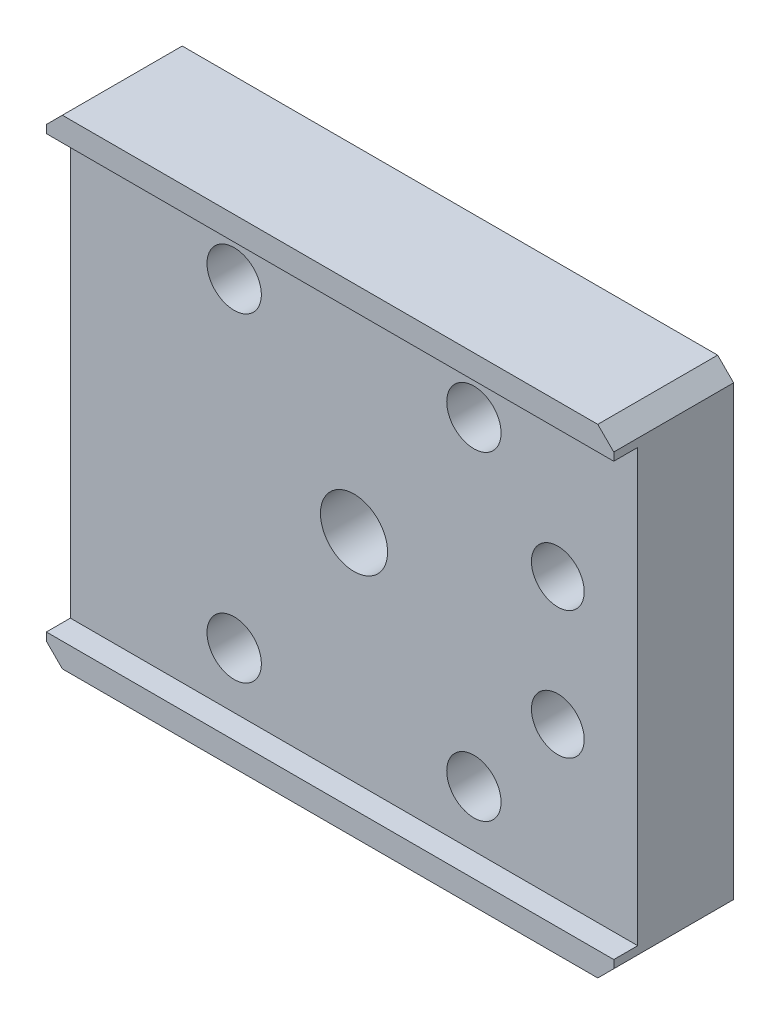
from build123d import *

# Parameters (mm, degrees)
SKETCH1_W                                           = 35.5
SKETCH1_H                                           = 30
BOSS_EXTRUDE1_DEPTH                                 = 5.25
SKETCH2_W                                           = 1.5
SKETCH2_H                                           = 27
CUT_EXTRUDE1_DEPTH                                  = 39.89489041
M5_TAPPED_HOLE1_D                                   = 4.2
M5_TAPPED_HOLE1_DEPTH                               = 12.4
M5_TAPPED_HOLE1_TIP                                 = 1.2618073
SKETCH14_OUTSIDE_W                                  = 47.03
SKETCH14_OUTSIDE_H                                  = 41.53
SKETCH14_OUTSIDE_W_2                                = 10
SKETCH14_OUTSIDE_H_2                                = 10
CUT_EXTRUDE4_DEPTH                                  = 3
CHAMFER1_SIZE                                       = 2
M4_TAPPED_HOLE3_D                                   = 3.3
M4_TAPPED_HOLE3_DEPTH                               = 10.1
M4_TAPPED_HOLE3_TIP                                 = 0.991420021
CHAMFER2_SIZE                                       = 1
CHAMFER3_SIZE                                       = 0.5
CBORE_FOR_M3_HEX_SOCKET_HEAD_CAP_SCREW1_D           = 3.4
CBORE_FOR_M3_HEX_SOCKET_HEAD_CAP_SCREW1_CBORE_D     = 6.5
CBORE_FOR_M3_HEX_SOCKET_HEAD_CAP_SCREW1_CBORE_DEPTH = 3.4
M3_TAPPED_HOLE1_D                                   = 2.5
M3_TAPPED_HOLE1_DEPTH                               = 7.5
M3_TAPPED_HOLE1_TIP                                 = 0.751075774


with BuildPart() as part:
    # Sketch1 → Boss-Extrude1 (new, symmetric)
    with BuildSketch(Plane.XY):
        Rectangle(SKETCH1_W, SKETCH1_H)
    extrude(amount=BOSS_EXTRUDE1_DEPTH, both=True)

    # Sketch2 → Cut-Extrude1 (cut, through all)
    with BuildSketch(Plane(origin=(17.75, 0, 0), x_dir=(0, 0, -1), z_dir=(1, 0, 0))):
        with Locations((-4.5, 0)):
            Rectangle(SKETCH2_W, SKETCH2_H)
    extrude(amount=-CUT_EXTRUDE1_DEPTH, mode=Mode.SUBTRACT)

    # M5 Tapped Hole1
    with Locations(Plane(origin=(0, 0, -5.25), x_dir=(-1, 0, 0), z_dir=(0, 0, -1))):
        with Locations((0, 0)):
            Hole(M5_TAPPED_HOLE1_D / 2, depth=M5_TAPPED_HOLE1_DEPTH)
            with Locations((0, 0, -(M5_TAPPED_HOLE1_DEPTH + M5_TAPPED_HOLE1_TIP / 2))):  # 118° drill point
                Cone(0, M5_TAPPED_HOLE1_D / 2, M5_TAPPED_HOLE1_TIP, mode=Mode.SUBTRACT)

    # Sketch14 outside → Cut-Extrude4 (cut)
    with BuildSketch(Plane(origin=(0, 0, -5.25), x_dir=(-1, 0, 0), z_dir=(0, 0, -1))):
        Rectangle(SKETCH14_OUTSIDE_W, SKETCH14_OUTSIDE_H)
        Rectangle(SKETCH14_OUTSIDE_W_2, SKETCH14_OUTSIDE_H_2, mode=Mode.SUBTRACT)
    extrude(amount=-CUT_EXTRUDE4_DEPTH, mode=Mode.SUBTRACT)

    # Chamfer1
    chamfer1_edges = [part.edges().sort_by_distance(p)[0] for p in [
        (5, 5, -3.75),
        (-5, 5, -3.75),
        (-5, -5, -3.75),
        (5, -5, -3.75),
    ]]
    chamfer(chamfer1_edges, length=CHAMFER1_SIZE)

    # M4 Tapped Hole3
    with Locations(Plane(origin=(0, 0, -2.25), x_dir=(-1, 0, 0), z_dir=(0, 0, -1))):
        with Locations((-12.75, 4), (-12.75, -4)):
            Hole(M4_TAPPED_HOLE3_D / 2, depth=M4_TAPPED_HOLE3_DEPTH)
            with Locations((0, 0, -(M4_TAPPED_HOLE3_DEPTH + M4_TAPPED_HOLE3_TIP / 2))):  # 118° drill point
                Cone(0, M4_TAPPED_HOLE3_D / 2, M4_TAPPED_HOLE3_TIP, mode=Mode.SUBTRACT)

    # Chamfer2
    chamfer2_edges = [part.edges().sort_by_distance(p)[0] for p in [
        (17.75, -15, 1.5),
        (-17.75, -15, 1.5),
        (-17.75, 15, 1.5),
        (17.75, 15, 1.5),
    ]]
    chamfer(chamfer2_edges, length=CHAMFER2_SIZE)

    # Chamfer3
    chamfer3_edges = [part.edges().sort_by_distance(p)[0] for p in [
        (-2.1, 0, -5.25),
        (5, 0, -5.25),
        (0, 5, -5.25),
        (0, -5, -5.25),
        (-5, 0, -5.25),
        (-4, -4, -5.25),
        (-4, 4, -5.25),
        (4, 4, -5.25),
        (4, -4, -5.25),
    ]]
    chamfer(chamfer3_edges, length=CHAMFER3_SIZE)

    # CBORE for M3 Hex Socket Head Cap Screw1 (through all)
    with Locations(Plane(origin=(0, 0, -2.25), x_dir=(-1, 0, 0), z_dir=(0, 0, -1))):
        with Locations((-7.5, 10), (7.5, 10), (7.5, -10), (-7.5, -10)):
            CounterBoreHole(CBORE_FOR_M3_HEX_SOCKET_HEAD_CAP_SCREW1_D / 2, CBORE_FOR_M3_HEX_SOCKET_HEAD_CAP_SCREW1_CBORE_D / 2, CBORE_FOR_M3_HEX_SOCKET_HEAD_CAP_SCREW1_CBORE_DEPTH)

    # M3 Tapped Hole1
    with Locations(Plane(origin=(-17.75, -2.75, 0), x_dir=(0, -1, 0), z_dir=(-1, 0, 0))):
        with Locations((3.25, 1.5), (-8.75, 1.5)):
            Hole(M3_TAPPED_HOLE1_D / 2, depth=M3_TAPPED_HOLE1_DEPTH)
            with Locations((0, 0, -(M3_TAPPED_HOLE1_DEPTH + M3_TAPPED_HOLE1_TIP / 2))):  # 118° drill point
                Cone(0, M3_TAPPED_HOLE1_D / 2, M3_TAPPED_HOLE1_TIP, mode=Mode.SUBTRACT)


solid = part.part
